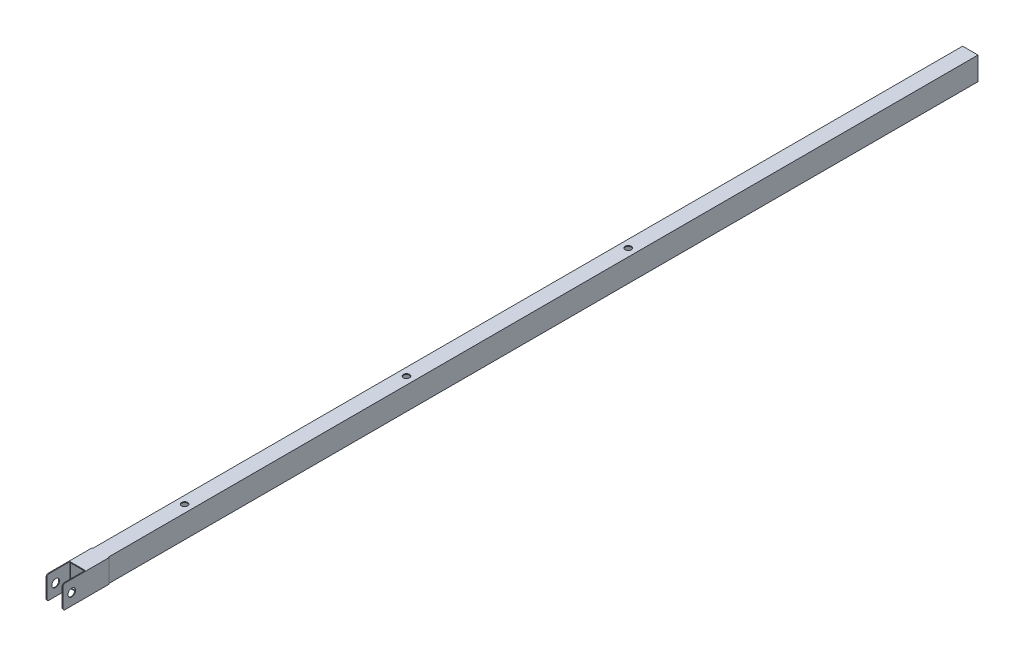
from build123d import *

# Parameters (mm, degrees)
SKETCH1_W           = 20
SKETCH1_H           = 30
SKETCH1_W_2         = 18
SKETCH1_H_2         = 28
BOSS_EXTRUDE1_DEPTH = 859
BOSS_EXTRUDE2_DEPTH = 1
SKETCH4_R           = 5
CUT_EXTRUDE1_DEPTH  = 890.778062216
SKETCH5_R           = 4
CUT_EXTRUDE2_DEPTH  = 890.753898558
SKETCH6_W           = 20
SKETCH6_H           = 30
SKETCH6_W_2         = 18
SKETCH6_H_2         = 28
BOSS_EXTRUDE3_DEPTH = 300


with BuildPart() as part:
    # Sketch1 → Boss-Extrude1 (new body)
    with BuildSketch(Plane.XY):
        with Locations((10, -15)):
            Rectangle(SKETCH1_W, SKETCH1_H)
        with Locations((10, -15)):
            Rectangle(SKETCH1_W_2, SKETCH1_H_2, mode=Mode.SUBTRACT)
    extrude(amount=BOSS_EXTRUDE1_DEPTH)

    # Sketch3 → Boss-Extrude2 (add)
    with BuildSketch(Plane.ZY):
        with BuildLine():
            Line((829, -30), (859, -30))
            Line((859, -30), (886, -30))
            ThreePointArc((886, -30), (888.121320344, -29.121320344), (889, -27))
            Line((889, -27), (889, -3))
            ThreePointArc((889, -3), (888.121320344, -0.878679656), (886, 0))
            Line((886, 0), (859, 0))
            Line((859, 0), (829, 0))
            Line((829, 0), (829, -30))
        make_face()
    boss_extrude2 = extrude(amount=BOSS_EXTRUDE2_DEPTH)

    # Mirror2: Boss-Extrude2 across plane
    add(boss_extrude2.mirror(Plane(origin=(10, 0, 0), x_dir=(0, 0, 1), z_dir=(1, 0, 0))))

    # Sketch4 → Cut-Extrude1 (cut, through all)
    with BuildSketch(Plane(origin=(21, 0, 0), x_dir=(0, 0, -1), z_dir=(1, 0, 0))):
        with Locations(Location((-877.5, -15, 0), (0, 0, 90))):
            Circle(SKETCH4_R)
    extrude(amount=-CUT_EXTRUDE1_DEPTH, mode=Mode.SUBTRACT)

    # Sketch5 → Cut-Extrude2 (cut, through all)
    with BuildSketch(Plane(origin=(0, 0, 0), x_dir=(1, 0, 0), z_dir=(0, 1, 0))):
        with Locations(Location((10, -144, 0), (0, 0, 270))):
            Circle(SKETCH5_R)
        with Locations(Location((10, -432, 0), (0, 0, 270))):
            Circle(SKETCH5_R)
        with Locations(Location((10, -720, 0), (0, 0, 270))):
            Circle(SKETCH5_R)
    extrude(amount=-CUT_EXTRUDE2_DEPTH, mode=Mode.SUBTRACT)

    # Sketch6 → Boss-Extrude3 (add)
    with BuildSketch(Plane(origin=(0, 0, 0), x_dir=(-1, 0, 0), z_dir=(0, 0, -1))):
        with Locations((-10, -15)):
            Rectangle(SKETCH6_W, SKETCH6_H)
        with Locations((-10, -15)):
            Rectangle(SKETCH6_W_2, SKETCH6_H_2, mode=Mode.SUBTRACT)
    extrude(amount=BOSS_EXTRUDE3_DEPTH)


solid = part.part
